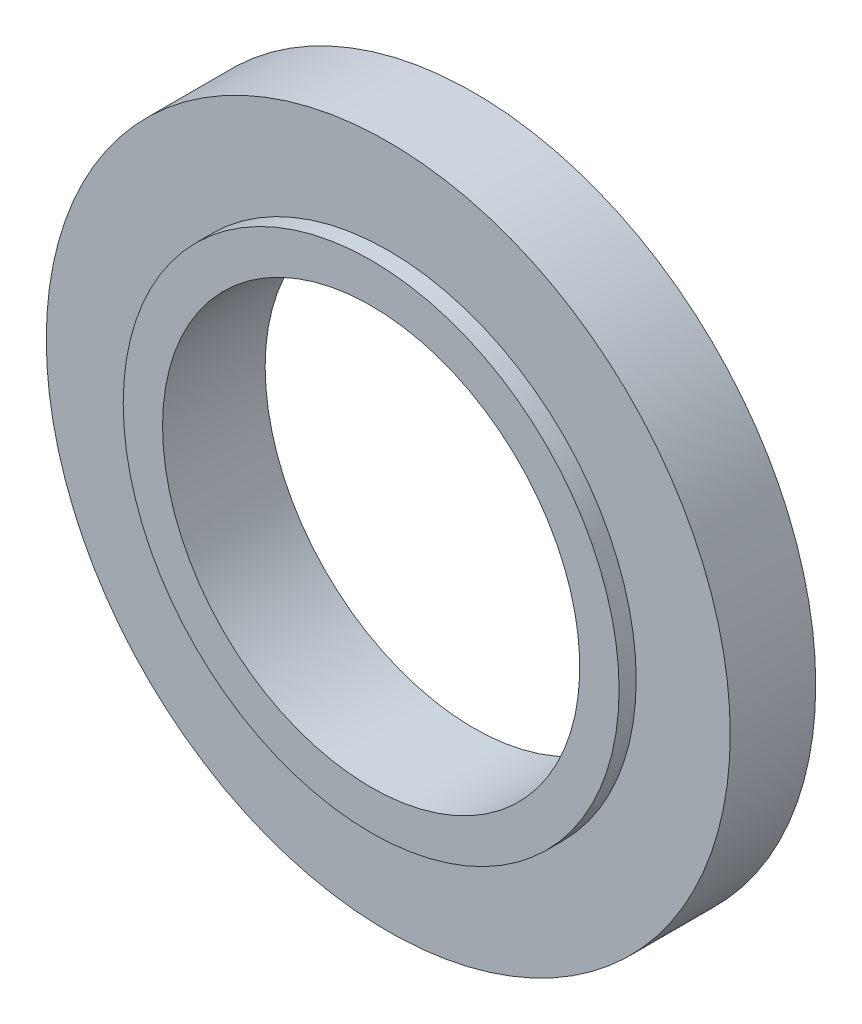
SolidWorks part; units mm, degrees
material "1023 碳钢板 (SS)"
ref_plane "Front Plane" through (0, 0, 0) normal (0, 0, 1) x (1, 0, 0)
ref_plane "Top Plane" through (0, 0, 0) normal (0, 1, 0) x (1, 0, 0)
ref_plane "Right Plane" through (0, 0, 0) normal (1, 0, 0) x (0, 0, -1)
ref_plane "Plane4" through (0, 0, 0) normal (0, -1, 0) x (1, 0, 0)
sketch "Sketch1" plane through (0, 0, 0) normal (0, -1, 0) x (1, 0, 0)
  line L0 (6.1, 1.5) -> (6.1, -1.5)
  line L1 (6.1, -1.5) -> (10, -1.5)
  line L2 (10, -1.5) -> (10, 1)
  line L3 (10, 1) -> (7.25, 1)
  line L4 (7.25, 1) -> (7.25, 1.5)
  line L5 (7.25, 1.5) -> (6.1, 1.5)
  line L6 (0, 1.5) -> (0, -1.5) construction
revolve "Revolve1" add sketch "Sketch1" angle 360 about L6
